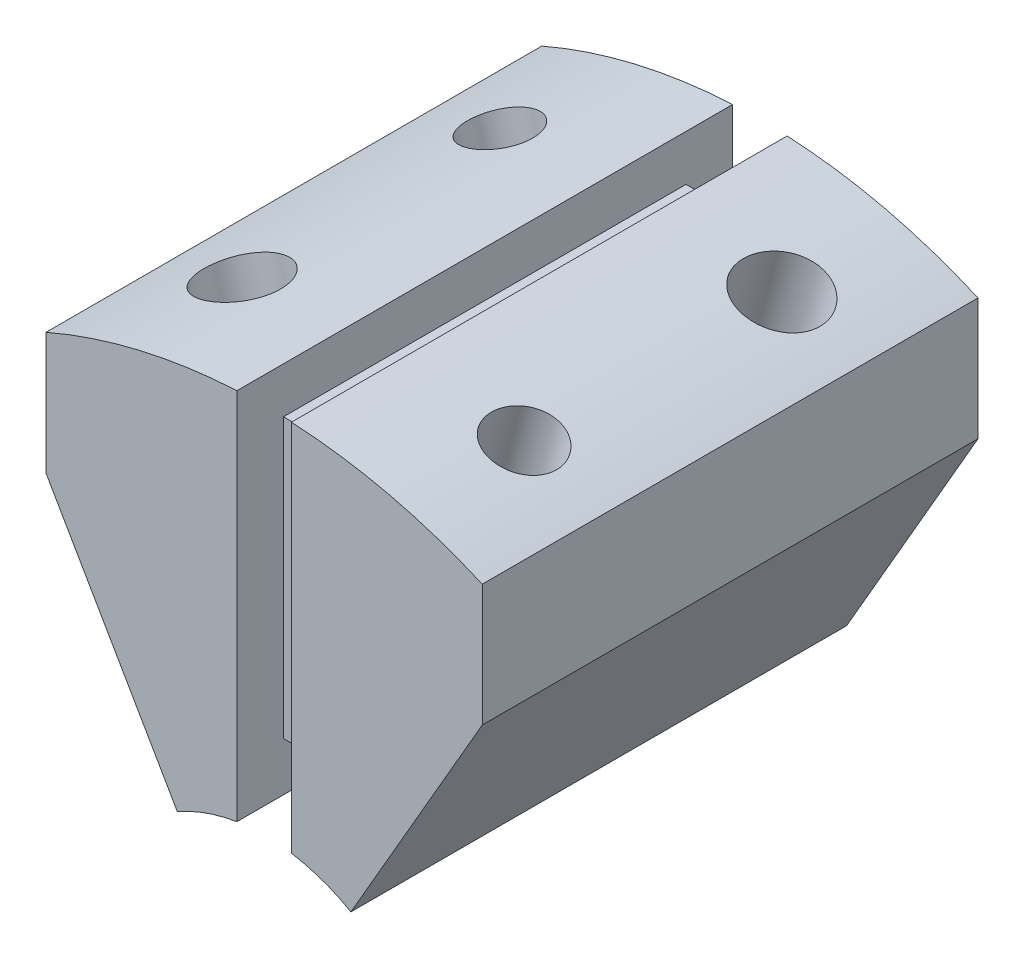
SolidWorks part; units mm, degrees
ref_plane "Front Plane" through (0, 0, 0) normal (0, 0, 1) x (1, 0, 0)
ref_plane "Top Plane" through (0, 0, 0) normal (0, 1, 0) x (1, 0, 0)
ref_plane "Right Plane" through (0, 0, 0) normal (1, 0, 0) x (0, 0, -1)
other "Configuration Table"
sketch "Sketch1" plane through (0, 0, 0) normal (0, 0, 1) x (1, 0, 0)
  line L0 (0, 0) -> (0, 30.181) construction
  line L1 (-8.75, 15.1554) -> (-22, 38.1051)
  line L2 (8.75, 15.1554) -> (22, 38.1051)
  line L3 (-22, 50.4083) -> (-22, 38.1051)
  line L4 (-2.75, 54.9312) -> (-2.75, 17.2826)
  line L5 (22, 50.4083) -> (22, 38.1051)
  line L6 (2.75, 54.9312) -> (2.75, 17.2826)
  line L9 (0, 0) -> (-8.75, 15.1554) construction
  line L10 (0, 0) -> (8.75, 15.1554) construction
  arc A1 (8.75, 15.1554) -> (2.75, 17.2826) centre (0, 0) ccw
  arc A2 (22, 50.4083) -> (2.75, 54.9312) centre (0, 0) ccw
  arc A3 (-2.75, 54.9312) -> (-22, 50.4083) centre (0, 0) ccw
  arc A4 (-2.75, 17.2826) -> (-8.75, 15.1554) centre (0, 0) ccw
  dimension "D1" = 55
  dimension "D2" = 17.5
  dimension "D8" = 30
  dimension "D3" = 30
  dimension "D4" = 22
  dimension "D5" = 2.75
extrude "Boss-Extrude1" add sketch "Sketch1" along normal mid plane 50
sketch "Sketch2" plane through (0, 0, 0) normal (0, 0, 1) x (1, 0, 0)
  line L0 (-2.75, 17.2826) -> (-2.75, 54.9312) construction
  line L1 (2.75, 22.2) -> (-2.75, 22.2)
  line L2 (2.75, 22.2) -> (2.75, 50.3)
  line L3 (2.75, 50.3) -> (-2.75, 50.3)
  line L4 (-2.75, 22.2) -> (-2.75, 50.3)
  line L5 (2.75, 22.2) -> (-2.75, 50.3) construction
  line L6 (2.75, 50.3) -> (-2.75, 22.2) construction
  point P0 (0, 36.25)
  dimension "D1" = 22.2
  dimension "D2" = 50.3
  dimension "D3" = 5.5
extrude "Boss-Extrude2" add sketch "Sketch2" along normal mid plane 40.6
ref_plane "Plane1" through (0, 0, 13) normal (0, 0, 1) x (1, 0, 0)
sketch "Sketch3" plane through (0, 0, 13) normal (0, 0, 1) x (1, 0, 0)
  line L0 (0, 0) -> (-14.235, 53.1259) construction
  line L1 (0, 0) -> (0, 31.6849) construction
  line L2 (0, 0) -> (14.235, 53.1259) construction
  arc A0 (-2.75, 54.9312) -> (-22, 50.4083) centre (0, 0) ccw construction
  dimension "D1" = 15
ref_plane "Plane2" through (0, 0, -13) normal (0, 0, 1) x (1, 0, 0)
sketch "Sketch4" plane through (0, 0, -13) normal (0, 0, 1) x (1, 0, 0)
  line L0 (0, 0) -> (14.235, 53.1259) construction
  line L1 (0, 0) -> (-14.235, 53.1259) construction
  line L2 (0, 0) -> (14.235, 53.1259) construction
  line L3 (0, 0) -> (-14.235, 53.1259) construction
hole_wizard "Ø8.0mm Blind Dowel Hole1" positions "3DSketch1" profile "Sketch5" hole size "Ø8.0" standard "GB"
sketch3d "3DSketch1"
  point P0 (-14.235, 53.1259, 13)
  point P2 (14.235, 53.1259, -13)
sketch "Sketch5" plane through (-14.235, 53.1259, 13) normal (0, 0, 1) x (-0.9659, -0.2588, 0)
  line L0 (0, 0) -> (0, 17.4034)
  line L1 (0, 17.4034) -> (4, 15)
  line L2 (4, 15) -> (4, 0)
  line L5 (4, 0) -> (0, 0)
  line L10 (0, 17.4034) -> (-4, 15) construction
  line L11 (0, -6.35) -> (0, 107.95) construction
  dimension "孔直径" = 8
  dimension "孔深度" = 15
  dimension "导头角度" = 118
hole_wizard "M8 Tapped Hole1" positions "3DSketch2" profile "Sketch6" tap size "M8" standard "GB"
sketch3d "3DSketch2"
  point P0 (-14.235, 53.1259, -13)
  point P2 (14.235, 53.1259, 13)
  point P5 (14.235, 53.1259, 13)
  point P7 (14.235, 53.1259, 13)
  point P11 (14.235, 53.1259, 13)
  point P13 (14.235, 53.1259, 13)
  point P15 (14.235, 53.1259, 13)
sketch "Sketch6" plane through (-14.235, 53.1259, -13) normal (0, 0, 1) x (-0.9659, -0.2588, 0)
  line L0 (0, 0) -> (0, 20.0429)
  line L1 (0, 20.0429) -> (3.4, 18)
  line L2 (3.4, 18) -> (3.4, 0)
  line L5 (3.4, 0) -> (0, 0)
  line L10 (0, 20.0429) -> (-3.4, 18) construction
  line L11 (0, -6.35) -> (0, 107.95) construction
  dimension "螺纹孔钻头直径" = 6.8
  dimension "螺纹孔钻头深度" = 18
  dimension "导头角度" = 118
cosmetic thread "Cosmetic Thread1" parameters "D1"=15, "D2"=8
cosmetic thread "Cosmetic Thread2" parameters "D1"=15, "D2"=8
cosmetic thread "Cosmetic Thread3" parameters "D1"=15, "D2"=8
